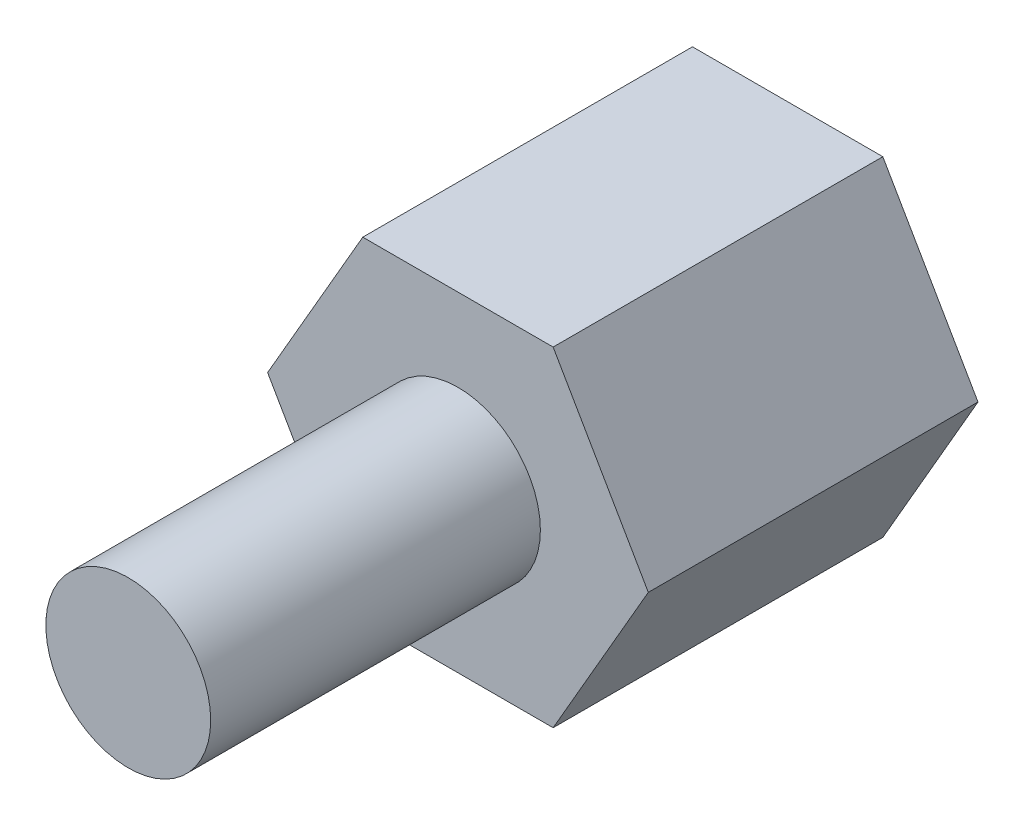
from build123d import *

# Parameters (mm, degrees)
EXTRUDE_1_DEPTH     = 6
SKETCH_2_R          = 1.5
EXTRUDE_2_DEPTH     = 6
SKETCH_3_R          = 1.5
CUT_EXTRUDE_1_DEPTH = 3


with BuildPart() as part:
    # 草图1 → 凸台-拉伸1 (new body)
    with BuildSketch(Plane.XY):
        Polygon((3.464101615, 0), (1.732050808, 3), (-1.732050808, 3), (-3.464101615, 0), (-1.732050808, -3), (1.732050808, -3), align=None)
    extrude(amount=EXTRUDE_1_DEPTH)

    # 草图2 → 凸台-拉伸2 (add)
    with BuildSketch(Plane.XY.offset(6)):
        Circle(SKETCH_2_R)
    extrude(amount=EXTRUDE_2_DEPTH)

    # 草图3 → 切除-拉伸1 (cut)
    with BuildSketch(Plane(origin=(0, 0, 0), x_dir=(-1, 0, 0), z_dir=(0, 0, -1))):
        with Locations(Location((0, 0, 0), (0, 0, 180))):
            Circle(SKETCH_3_R)
    extrude(amount=-CUT_EXTRUDE_1_DEPTH, mode=Mode.SUBTRACT)


solid = part.part
